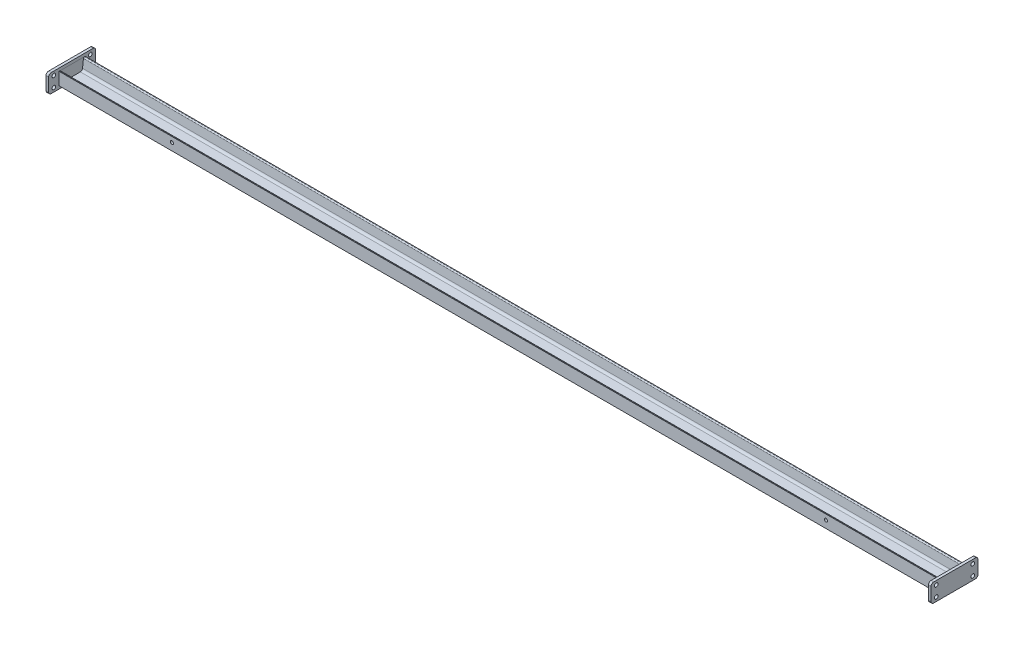
SolidWorks part; units mm, degrees
material "普通碳钢"
ref_plane "Front Plane" through (0, 0, 0) normal (0, 0, 1) x (1, 0, 0)
ref_plane "Top Plane" through (0, 0, 0) normal (0, 1, 0) x (1, 0, 0)
ref_plane "Right Plane" through (0, 0, 0) normal (1, 0, 0) x (0, 0, -1)
other "Configuration Table"
sketch "Sketch1" plane through (0, 0, 0) normal (0, 1, 0) x (1, 0, 0)
  line L0 (-1685.5, 0) -> (1685.5, 0)
  dimension "D1" = 3371
other "Gb／t707-1988 Hot-Rolled Channel 10(1)"
ref_plane "Plane1" through (-1685.5, 0, -50) normal (1, 0, 0) x (0, 1, 0)
sketch "Sketch13" plane through (-1685.5, 0, -50) normal (1, 0, 0) x (0, 1, 0)
  line L0 (48, 100) -> (0, 100)
  line L1 (48, 0) -> (0, 0)
  line L2 (0, 100) -> (0, 0)
  line L3 (-9.5694, 50) -> (49.7414, 50) construction
  line L4 (5.3, 81.6026) -> (5.3, 18.3974)
  line L5 (48, 0) -> (48, 2.4743)
  line L6 (48, 100) -> (48, 97.5257)
  line L7 (12.9115, 9.944) -> (44.239, 6.6513)
  line L17 (12.9115, 90.056) -> (44.239, 93.3487)
  arc A0 (44.239, 93.3487) -> (48, 97.5257) centre (43.8, 97.5257) ccw
  arc A1 (44.239, 6.6513) -> (48, 2.4743) centre (43.8, 2.4743) cw
  arc A2 (5.3, 18.3974) -> (12.9115, 9.944) centre (13.8, 18.3974) ccw
  arc A10 (5.3, 81.6026) -> (12.9115, 90.056) centre (13.8, 81.6026) cw
  point P6 (0, 0)
  point P8 (0, 50)
  point P9 (5.3, 25.8841)
  point P10 (24, 100)
  point P13 (48, 93.744)
  point P14 (26.65, 91.5)
  point P19 (5.3, 50)
sketch "Sketch3" plane through (-1685.5, 0, 0) normal (-1, 0, 0) x (0, 0, 1)
  line L0 (50, 0) -> (-50, 48) construction
  line L5 (-80, 59) -> (80, 59)
  line L6 (-90, 49) -> (-90, -1)
  line L9 (-80, -11) -> (80, -11)
  line L10 (90, 49) -> (90, -1)
  line L11 (-90, 59) -> (90, -11) construction
  line L12 (-90, -11) -> (90, 59) construction
  line L13 (0, 24) -> (-121.7093, 24) construction
  line L14 (0, 24) -> (0, 93.146) construction
  arc A16 (-90, -1) -> (-80, -11) centre (-80, -1) ccw
  arc A17 (80, -11) -> (90, -1) centre (80, -1) ccw
  arc A18 (80, 59) -> (90, 49) centre (80, 49) cw
  arc A19 (-80, 59) -> (-90, 49) centre (-80, 49) ccw
  circle A20 centre (-70, 44) radius 7
  circle A21 centre (-70, 4) radius 7
  circle A22 centre (70, 4) radius 7
  circle A23 centre (70, 44) radius 7
  point P3 (0, 24)
  dimension "D3" = 10
  dimension "D4" = 40
  dimension "D5" = 20
  dimension "D6" = 14
  dimension "D1" = 70
  dimension "D2" = 180
extrude "Boss-Extrude1" add sketch "Sketch3" along normal blind 10 separate body
sketch "Sketch8" plane through (-1685.5, 0, 0) normal (1, 0, 0) x (0, 0, -1)
  line L0 (50, 0) -> (50, 48) construction
  line L1 (50, 0) -> (-50, 0)
  line L2 (50, 0) -> (50, 48)
  line L3 (50, 48) -> (-50, 48)
  line L4 (-50, 0) -> (-50, 48)
  line L5 (-50, 0) -> (50, 0) construction
split line "Split Line1"
mirror "Mirror3" about plane through (0, 0, 0) normal (1, 0, 0) of bodies 109 107
sketch "Sketch9" plane through (0, 0, 50) normal (0, 0, -1) x (-1, 0, 0)
  line L0 (0, 0) -> (0, 48) construction
  line L1 (-1685.5, 48) -> (1685.5, 48) construction
  line L2 (-1253, 28) -> (1253, 28) construction
  circle A0 centre (-1253, 28) radius 6
  circle A1 centre (1253, 28) radius 6
  point P8 (0, 28)
  dimension "D3" = 12
  dimension "D1" = 20
  dimension "D2" = 2506
extrude "Cut-Extrude1" cut sketch "Sketch9" along normal blind 10
equation "\"RI@Sketch13\"= \"D1@Sketch13\""
equation "\"D3@Sketch13\"=  ( \"BF@Sketch13\" - \"D6@Sketch13\" )  / 2"
